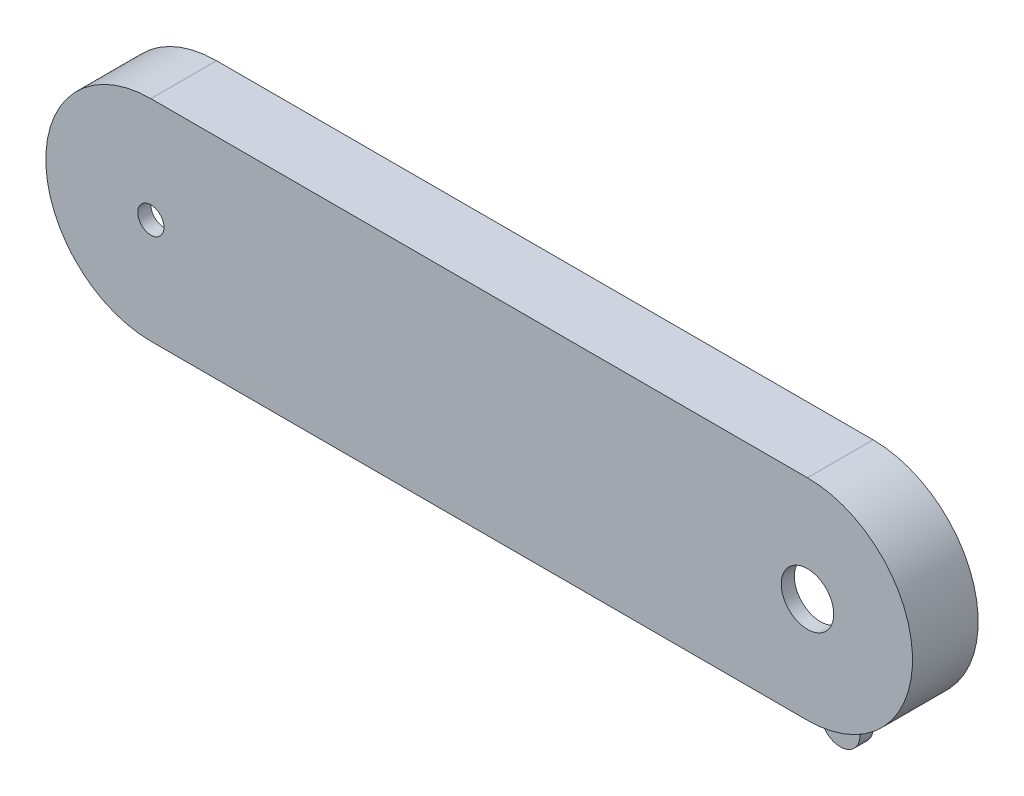
SolidWorks part; units mm, degrees
ref_plane "前视基准面" through (0, 0, 0) normal (0, 0, 1) x (1, 0, 0)
ref_plane "上视基准面" through (0, 0, 0) normal (0, 1, 0) x (1, 0, 0)
ref_plane "右视基准面" through (0, 0, 0) normal (1, 0, 0) x (0, 0, -1)
sketch "草图1" plane through (0, 0, 0) normal (0, 0, 1) x (1, 0, 0)
  line L0 (0, 80) -> (-500, 80)
  line L2 (-500, -80) -> (0, -80)
  arc A0 (0, -80) -> (0, 80) centre (0, 0) ccw
  circle A2 centre (0, 0) radius 20
  arc A7 (-500, 80) -> (-500, -80) centre (-500, 0) ccw
  circle A8 centre (-500, 0) radius 10
extrude "凸台-拉伸1" add sketch "草图1" along normal blind 10
sketch "草图2" plane through (0, 0, 0) normal (0, 0, -1) x (-1, 0, 0)
  line L0 (0, -70) -> (500, -70)
  line L1 (500, 70) -> (0, 70)
  line L2 (0, -80) -> (500, -80)
  line L3 (500, 80) -> (0, 80)
  line L4 (0, -80) -> (500, -80)
  line L5 (500, 80) -> (0, 80)
  arc A0 (500, -70) -> (500, 70) centre (500, 0) ccw
  arc A1 (0, 70) -> (0, -70) centre (0, 0) ccw
  arc A2 (0, 80) -> (0, -80) centre (0, 0) ccw
  arc A3 (500, -80) -> (500, 80) centre (500, 0) ccw
  arc A4 (0, 80) -> (0, -80) centre (0, 0) ccw
  arc A5 (500, -80) -> (500, 80) centre (500, 0) ccw
  dimension "D1" = 0
  dimension "D2" = 10
extrude "凸台-拉伸2" add sketch "草图2" along normal blind 40
sketch "草图4" plane through (0, 0, -40) normal (0, 0, -1) x (-1, 0, 0)
  line L0 (0, -80) -> (500, -80) construction
  line L5 (30, -110) -> (30, -80)
  line L6 (0, -80) -> (30, -80)
  line L7 (0, -110) -> (0, -80)
  circle A2 centre (15, -110) radius 5
  arc A3 (30, -110) -> (0, -110) centre (15, -110) cw
  dimension "D2" = 10
  dimension "D1" = 30
  dimension "D3" = 30
  dimension "D5" = 15
extrude "凸台-拉伸3" add sketch "草图4" against normal blind 10
